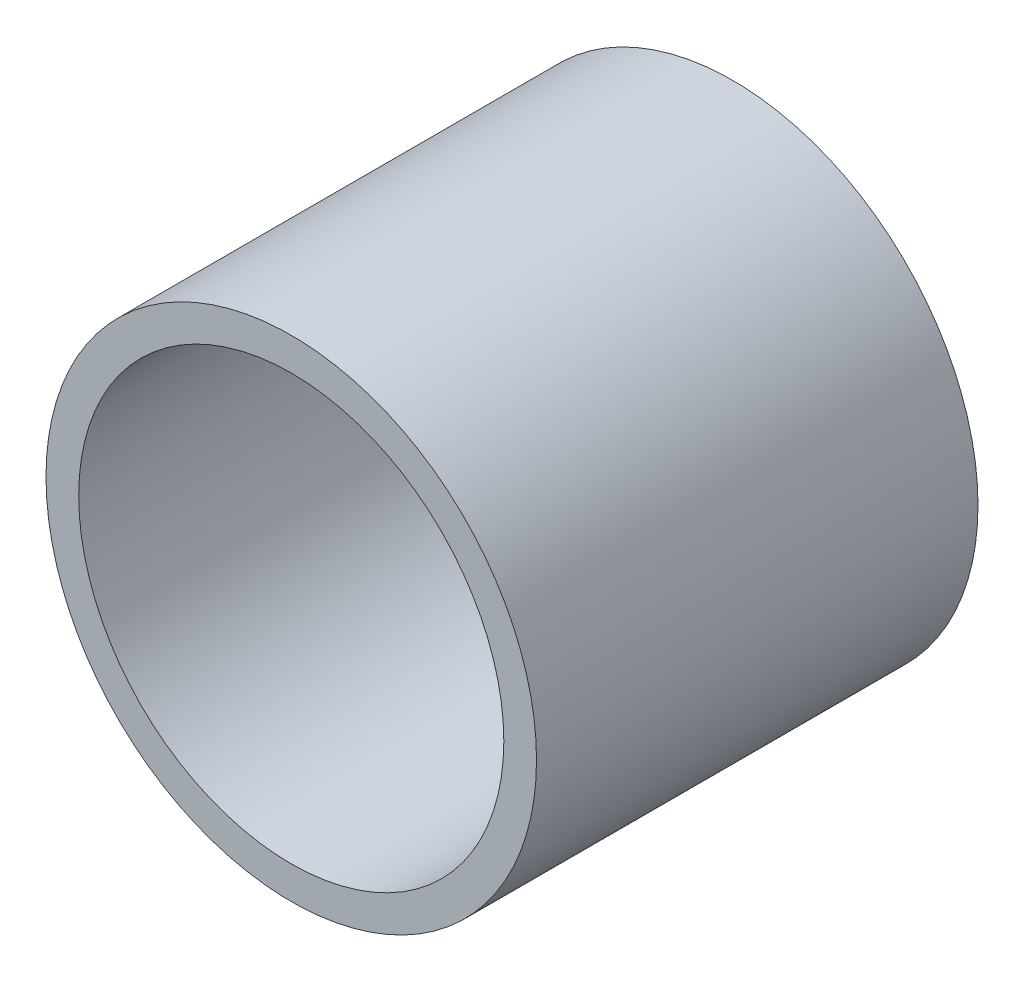
SolidWorks part; units mm, degrees
material "AISI 1045 钢，冷拔"
ref_plane "Front Plane" through (0, 0, 0) normal (0, 0, 1) x (1, 0, 0)
ref_plane "Top Plane" through (0, 0, 0) normal (0, 1, 0) x (1, 0, 0)
ref_plane "Right Plane" through (0, 0, 0) normal (1, 0, 0) x (0, 0, -1)
sketch "Sketch1" plane through (0, 0, 0) normal (0, 0, 1) x (1, 0, 0)
  circle A0 centre (0, 0) radius 13
  circle A1 centre (0, 0) radius 15
  dimension "D1" = 26
  dimension "D2" = 30
extrude "Boss-Extrude1" add sketch "Sketch1" along normal blind 27
